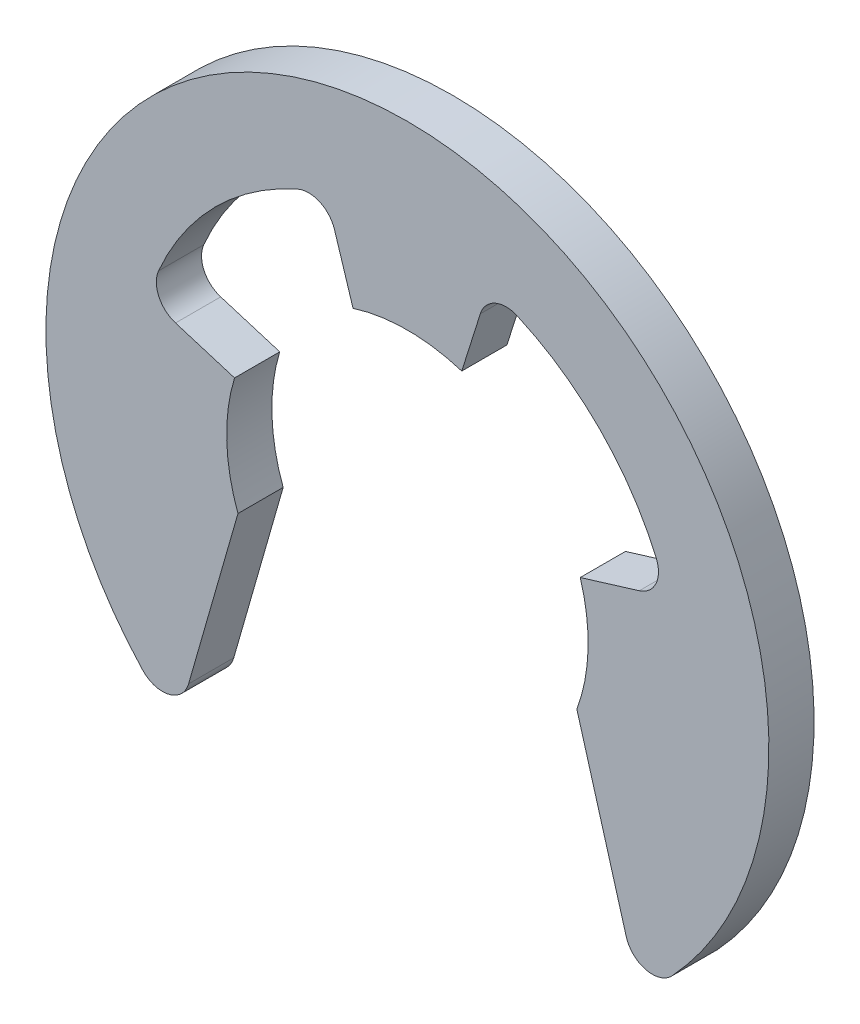
from build123d import *

# Parameters (mm, degrees)
EXTRUDE1_DEPTH = 1


with BuildPart() as part:
    # Sketch1 → Extrude1 (new body)
    with BuildSketch(Plane.XY):
        with BuildLine():
            Line((3.75, -1.391941091), (4.843037844, -5.203817057))
            ThreePointArc((4.843037844, -5.203817057), (5.280177605, -5.621964438), (5.859237689, -5.446956371))
            ThreePointArc((5.859237689, -5.446956371), (0, 8), (-5.859237689, -5.446956371))
            ThreePointArc((-5.859237689, -5.446956371), (-5.280177605, -5.621964438), (-4.843037844, -5.203817057))
            Line((-4.843037844, -5.203817057), (-3.75, -1.391941091))
            ThreePointArc((-3.75, -1.391941091), (-3.998276385, -0.11741359), (-3.825219024, 1.169486819))
            Line((-3.825219024, 1.169486819), (-5.13206986, 1.569031215))
            ThreePointArc((-5.13206986, 1.569031215), (-5.501268007, 1.891044768), (-5.507385374, 2.380904521))
            ThreePointArc((-5.507385374, 2.380904521), (-4.261112254, 4.224088347), (-2.428874258, 5.486398622))
            ThreePointArc((-2.428874258, 5.486398622), (-1.938979773, 5.484556266), (-1.613756661, 5.11818224))
            Line((-1.613756661, 5.11818224), (-1.202823198, 3.814867803))
            ThreePointArc((-1.202823198, 3.814867803), (0, 4), (1.202823198, 3.814867803))
            Line((1.202823198, 3.814867803), (1.613756661, 5.11818224))
            ThreePointArc((1.613756661, 5.11818224), (1.938979773, 5.484556266), (2.428874258, 5.486398622))
            ThreePointArc((2.428874258, 5.486398622), (4.261112254, 4.224088347), (5.507385374, 2.380904521))
            ThreePointArc((5.507385374, 2.380904521), (5.501268007, 1.891044768), (5.13206986, 1.569031215))
            Line((5.13206986, 1.569031215), (3.825219024, 1.169486819))
            ThreePointArc((3.825219024, 1.169486819), (3.998276385, -0.11741359), (3.75, -1.391941091))
        make_face()
    extrude(amount=EXTRUDE1_DEPTH)


solid = part.part
